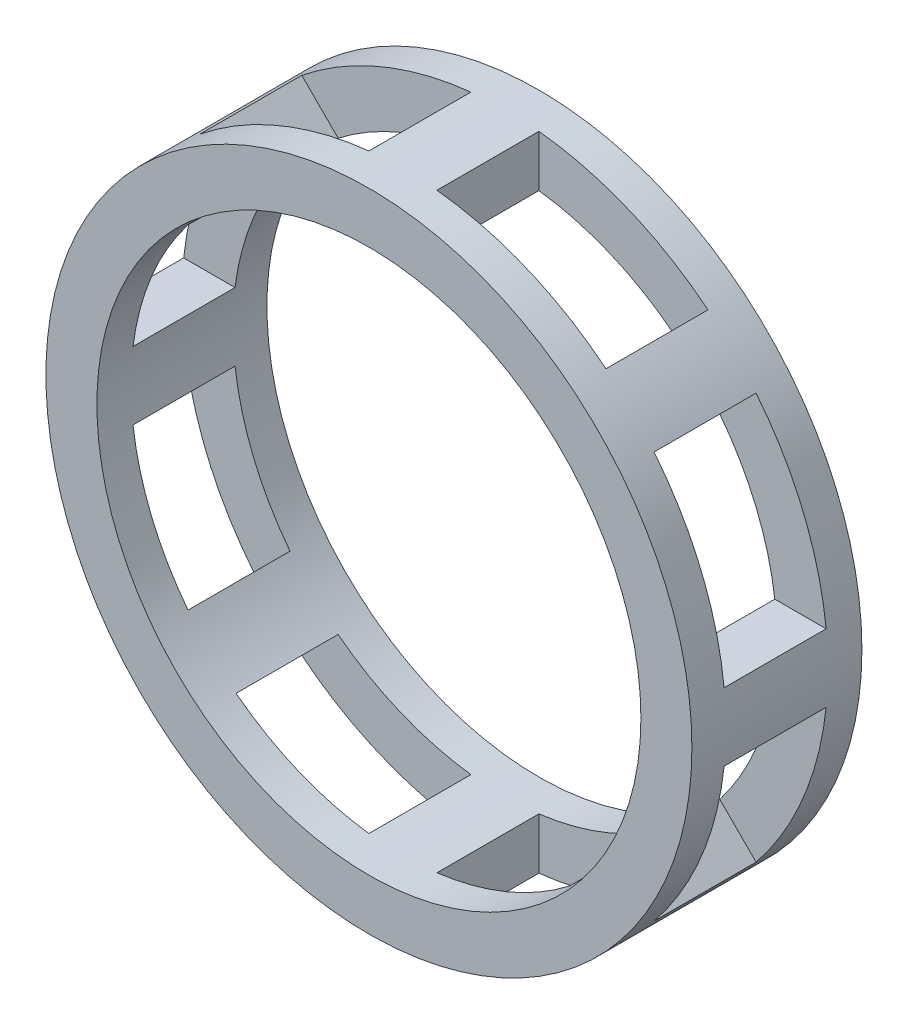
SolidWorks part; units mm, degrees
ref_plane "Front Plane" through (0, 0, 0) normal (0, 0, 1) x (1, 0, 0)
ref_plane "Top Plane" through (0, 0, 0) normal (0, 1, 0) x (1, 0, 0)
ref_plane "Right Plane" through (0, 0, 0) normal (1, 0, 0) x (0, 0, -1)
other "Configuration Table"
sketch "Sketch1" plane through (0, 0, 0) normal (0, 0, 1) x (1, 0, 0)
  circle A0 centre (-599.8842, -90) radius 80
  circle A1 centre (-599.8842, -90) radius 95
extrude "Boss-Extrude1" add sketch "Sketch1" along normal blind 50
sketch "Sketch2" plane through (0, 0, 50) normal (0, 0, 1) x (1, 0, 0)
  line L0 (-659.6151, -163.873) -> (-526.0112, -30.2691)
  line L1 (-505.412, -100) -> (-694.3564, -100)
  line L2 (-505.412, -100) -> (-505.412, -80)
  line L3 (-505.412, -80) -> (-694.3564, -80)
  line L4 (-694.3564, -100) -> (-694.3564, -80)
  line L5 (-505.412, -100) -> (-694.3564, -80) construction
  line L6 (-505.412, -80) -> (-694.3564, -100) construction
  line L7 (-589.8842, -184.4722) -> (-609.8842, -184.4722)
  line L8 (-589.8842, -184.4722) -> (-589.8842, 4.4722)
  line L9 (-589.8842, 4.4722) -> (-609.8842, 4.4722)
  line L10 (-609.8842, -184.4722) -> (-609.8842, 4.4722)
  line L11 (-589.8842, -184.4722) -> (-609.8842, 4.4722) construction
  line L12 (-589.8842, 4.4722) -> (-609.8842, -184.4722) construction
  line L13 (-673.7572, -149.7309) -> (-540.1533, -16.127)
  line L14 (-694.3564, -100) -> (-505.412, -100)
  line L15 (-694.3564, -80) -> (-505.412, -80)
  line L16 (-673.7572, -30.2691) -> (-540.1533, -163.873)
  line L17 (-659.6151, -16.127) -> (-526.0112, -149.7309)
  line L18 (-609.8842, 4.4722) -> (-609.8842, -184.4722)
  line L19 (-589.8842, 4.4722) -> (-589.8842, -184.4722)
  line L20 (-540.1533, -16.127) -> (-673.7572, -149.7309)
  line L21 (-526.0112, -30.2691) -> (-659.6151, -163.873)
  line L22 (-505.412, -80) -> (-694.3564, -80)
  line L23 (-505.412, -100) -> (-694.3564, -100)
  line L24 (-526.0112, -149.7309) -> (-659.6151, -16.127)
  line L25 (-540.1533, -163.873) -> (-673.7572, -30.2691)
  circle A0 centre (-599.8842, -90) radius 80
  circle A1 centre (-599.8842, -90) radius 95
  point P42 (-599.8842, -90)
  circle M4 centre (-599.8842, -90) radius 95
  circle M5 centre (-599.8842, -90) radius 80
  dimension "D1" = 20
  dimension "D2" = 8
extrude "Cut-Extrude1" cut sketch "Sketch2" against normal blind 30 from offset 10 contours L13 L1 M5 | L13 L1 M4 M5 | L10 L0 M5 | L10 L0 M4 M5 | L16 L8 M5 M4 | L16 L8 M5 | L1 L17 M5 | L17 L1 M5 M4 | L3 L0 M5 | L3 L0 M4 M5 | L8 L13 M5 | L13 L8 M5 M4 | L17 L10 M5 | L17 L10 M4 M5 | L16 L3 M4 M5 | L16 L15 M5 | A0
